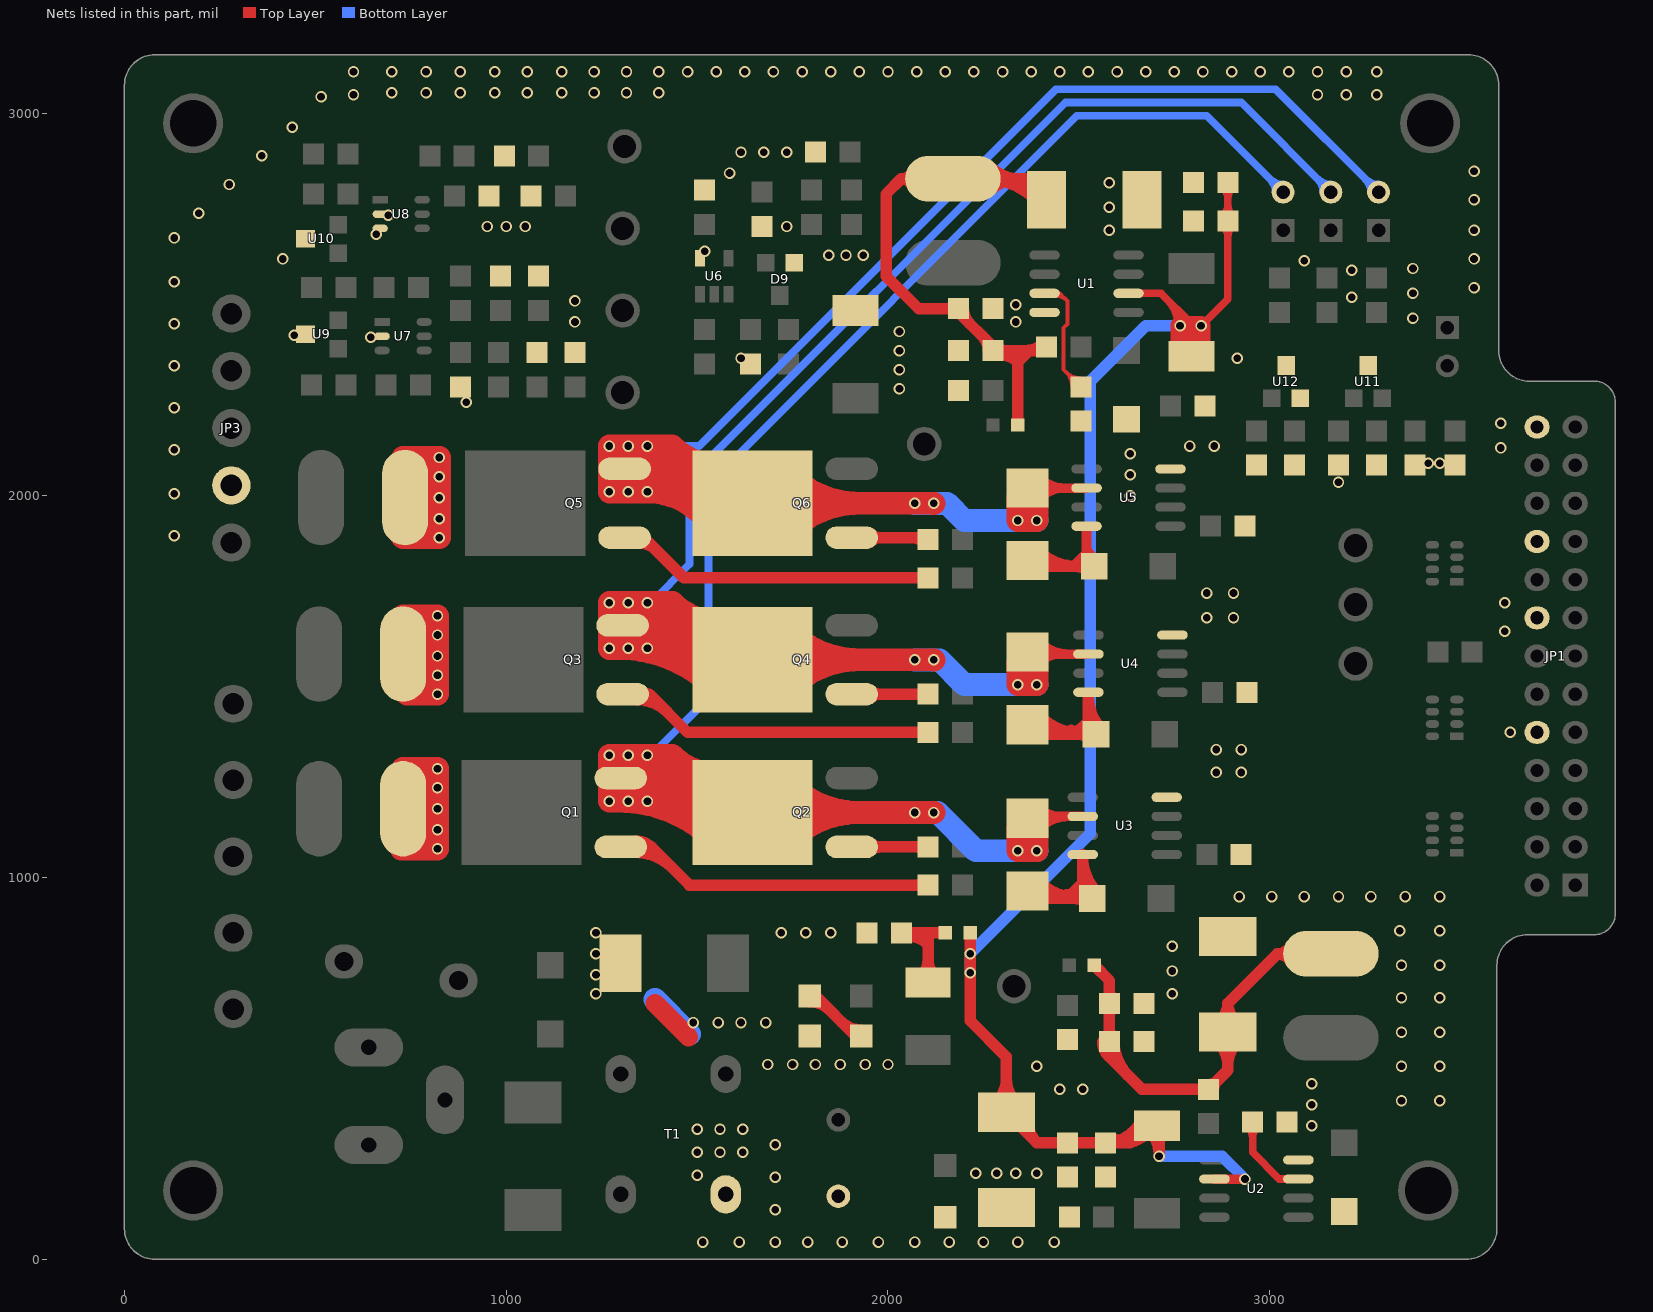
[diagram p0: the nets of this part, all layers, seen from the top]
# Altium PCB MISC103926.PcbDoc (part 2 of 4)
Units mil, origin at the board's own origin, x right, y up, seen from the top; angles counter-clockwise.
Board outline 3905 x 3155 mil, 4 copper layers (Top Layer, GND1, GND2, Bottom Layer); 132 components, 84 nets, 362 pads, 268 vias.

## Via types
v1: diameter 30, hole 20, Top Layer to Bottom Layer, 268 vias

## Nets (pads, with @x,y where several pads share a name; then routed paths per layer and width w, separated by ;. In a path a pad name is that pad's centre, name@x,y a point inside that pad or via, vN(x,y) a via of type N, cw(c..) or ccw(c..) an arc to the next point about the centre after c; other vN are vias at no path point) (continued)
GND: C2.2 C3.2 C4.2 C5.2 C6.2 C7.2 C8.2 C9.2 C10.2 C11.2 C12.2 C13.2 C14.2 C15.2 C16.2 C17.2 C19.2 C20.1 C21.1 C22.1 C26.1 C27.1 C28.2 C29.2 C30.2 C31.1 C32.2 C33.2 C34.2 C35.1 C36.1 C37.1 D3.2 D4.2 D5.2 D9.1 D10.2 JP1.10 JP1.16 JP1.20 JP1.26 JP3.2 R3.2 R5.2 R16.2 R19.1 R20.1 R21.1 R22.1 R32.2 R33.2 R34.2 T1.2 U1.4 U2.4 U3.4 U4.4 U5.4 U6.5 U7.2 U8.2 U8.3 U9.3 U10.3 U11.3 U12.2 U12.3 | length 352.7
  Top Layer w10: v1(645,2415) 647.6,2417.6 U7.2@675,2417.6 ccw(c675,2385.58) v1@652.14,2408 ; v1@652.07,2422.07 ccw(c662.87,2432.87) U7.2@662.87,2417.6 ; U7.2@661.46,2414.06 ccw(c652.93,2405.53) 652.93,2417.6 ccw(c652.93,2429.67) U7.2@661.46,2421.13
  Top Layer w50: 1390,670 1477.5,582.5
  Top Layer w60: C5.2@2285,125 C5.2@2295,135
  Bottom Layer w60: 1390,680 1480,590
  other v1: 1515,45 1610,45 1705,45 1790,45 1880,45 1975,45 2070,45 2160,45 2250,45 2340,45 2435,45 1705,130 1705,215 1500,220 2230,225 2285,225 2335,225 2390,225 1500,280 1560,280 1620,280 1705,300 1500,340 1560,340 1620,340 3110,350 3110,405 3345,415 3445,415 2450,445 2510,445 3110,460 2390,505 3345,505 3445,505 1685,510 1750,510 1810,510 1875,510 1940,510 2000,510 3345,595 3445,595 1490,620 1555,620 1615,620 1680,620 3345,685 3445,685 1235,695 2745,695 1235,745 2745,755 3345,770 3445,770 1235,800 2745,820 1235,855 1720,855 1785,855 1850,855 3340,860 3445,860 2920,950 3005,950 3090,950 3180,950 3265,950 3355,950 3445,950 2860,1275 2925,1275 2860,1335 2925,1335 3630,1380 3615,1645 2835,1680 2905,1680 3615,1720 2835,1745 2905,1745 130,1895 2635,2000 130,2005 3180,2035 2635,2055 3415,2085 3445.5,2085 2635,2110 130,2120 3605,2125 2790,2130 2855,2130 3605,2190 130,2230 895,2245 2030,2280 2030,2330 130,2340 1615,2360 2915,2360 2030,2380 445,2420 2030,2430 130,2450 1180,2455 2335,2455 3375,2465 2335,2500 1180,2510 3215,2520 3375,2530 3535,2545 130,2560 3215,2590 3375,2595 3090,2615 415,2620 3535,2620 1845,2630 1890,2630 1935,2630 1520,2640 130,2675 660,2685 2580,2695 3535,2695 950,2705 1000,2705 1050,2705 1735,2705 690.87,2734.06 195,2740 2580,2755 3535,2775 275,2815 2580,2820 1585,2845 3535,2850 360,2890 1615,2900 1675,2900 1735,2900 440,2965 515,3045 600,3050 3125,3050 3200,3050 3280,3050 700,3055 790,3055 880,3055 970,3055 1055,3055 1145,3055 1230,3055 1315,3055 1400,3055 600,3110 700,3110 790,3110 880,3110 970,3110 1055,3110 1145,3110 1230,3110 1315,3110 1400,3110 1475,3110 1550,3110 1625,3110 1700,3110 1775,3110 1850,3110 1925,3110 2000,3110 2075,3110 2150,3110 2225,3110 2300,3110 2375,3110 2450,3110 2525,3110 2600,3110 2675,3110 2750,3110 2825,3110 2900,3110 2975,3110 3050,3110 3125,3110 3200,3110 3280,3110
GT_UH: Q1.1 R9.2 | length 1101.2
  Top Layer w30: Q1.1@1300,1080 1380,1080 1480,980 R9.2@2105,980 ; Q1.1@1339.37,1065.47 cw(c1339.37,932.31) 1433.53,1026.47 ; Q1.1@1339.37,1095.47 cw(c1339.37,1034.73) 1382.32,1077.68 ; Q1.1@1349.64,1069.73 cw(c1374.44,1044.93) 1374.44,1080 cw(c1374.44,1115.07) Q1.1@1349.64,1090.27 ; R9.2@2096.16,971.16 ccw(c2074.82,949.82) 2074.82,980 ccw(c2074.82,1010.18) R9.2@2096.16,988.84
GT_UL: Q2.1 R10.2 | length 302.5
  Top Layer w30: Q2.1@1905,1080 R10.2@2105,1080 ; Q2.1@1954.64,1069.73 cw(c1979.44,1044.93) 1979.44,1080 cw(c1979.44,1115.07) Q2.1@1954.64,1090.27 ; R10.2@2096.16,1071.16 ccw(c2074.82,1049.82) 2074.82,1080 ccw(c2074.82,1110.18) R10.2@2096.16,1088.84
GT_VH: Q3.1 R11.2 | length 1018.8
  Top Layer w30: Q3.1@1305,1480 1375,1480 ; Q3.1@1344.37,1465.47 cw(c1344.37,1356.45) 1421.46,1433.54 ; Q3.1@1355.62,1470.81 cw(c1375,1454.97) 1375,1480 ; Q3.1@1355.62,1489.19 ccw(c1375,1505.02) 1375,1480 ; R11.2@2096.16,1371.16 ccw(c2074.82,1349.82) 2074.82,1380 ccw(c2074.82,1410.18) R11.2@2096.16,1388.84 ; R11.2@2105,1380 1475,1380 1375,1480
GT_VL: Q4.1 R12.2 | length 302.5
  Top Layer w30: Q4.1@1905,1480 R12.2@2105,1480 ; Q4.1@1954.64,1469.73 cw(c1979.44,1444.93) 1979.44,1480 cw(c1979.44,1515.07) Q4.1@1954.64,1490.27 ; R12.2@2096.16,1471.16 ccw(c2074.82,1449.82) 2074.82,1480 ccw(c2074.82,1510.18) R12.2@2096.16,1488.84
GT_WH: Q5.1 R13.2 | length 933.6
  Top Layer w30: Q5.1@1310,1890 1360,1890 1465,1785 R13.2@2105,1785 ; Q5.1@1349.37,1875.47 cw(c1349.37,1814.73) 1392.32,1857.68 ; R13.2@2096.16,1776.16 ccw(c2074.82,1754.82) 2074.82,1785 ccw(c2074.82,1815.18) R13.2@2096.16,1793.84
GT_WL: Q6.1 R14.2 | length 294.3
  Top Layer w20: R14.2@2100,1890 R14.2@2105,1885
  Top Layer w30: Q6.1@1905,1890 R14.2@2100,1890 ; Q6.1@1954.64,1879.73 cw(c1979.44,1854.93) 1979.44,1890 cw(c1979.44,1925.07) Q6.1@1954.64,1900.27 ; 2062.75,1890 cw(c2062.75,1842.75) R14.2@2096.16,1876.16
MT_PU: C23.2 J1.2 L6.1 Q1.3 Q2.2 U3.6 | length 9709.6
  Top Layer w25: C23.2@2370,1160 U3.6@2510,1160 ; C23.2@2396.29,1127.65 cw(c2474.39,1049.54) U3.6@2474.39,1160 ; C23.2@2396.29,1182.35 ccw(c2450.25,1236.31) 2450.25,1160
  Top Layer w50: C23.2@2340,1130 C23.2@2365,1155 C23.2@2390,1130
  Top Layer w60: L6.1@725,1075 v1(820,1075) ; L6.1@730,1285 v1(820,1285) ; L6.1@743.07,1088 cw(c772.39,1027.4) v1(820,1075) ; L6.1@743.07,1272 ccw(c772.4,1332.6) v1(820,1285) ; L6.1@751.21,1158.79 cw(c802.43,1107.57) 802.43,1180 cw(c802.43,1252.43) L6.1@751.21,1201.21 ; L6.1@759.08,1122.38 ccw(c820,1137.85) v1(820,1075) ; L6.1@759.08,1237.62 cw(c820,1222.15) v1(820,1285) ; L6.1@760.25,1134.75 ccw(c820,1194.5) 820,1110 ; L6.1@760.25,1225.25 cw(c820,1165.5) 820,1250 ; 805.5,1128.85 ccw(c859.51,1114.51) v1(820,1075) ; 805.5,1231.15 cw(c859.51,1245.49) v1(820,1285) ; 805.74,1175.33 cw(c861.43,1193.56) v1(820,1235) L6.1@765,1180 ; 805.74,1184.67 ccw(c861.43,1166.44) v1(820,1125) L6.1@765,1180 ; v1(820,1180) L6.1@730,1180 ; 1293.03,1200 cw(c1293.03,837.87) Q2.2@1549.09,1093.93 ; Q1.3@1309.68,1260.32 Q1.3@1300,1260.32 Q1.3@1310.32,1260.32 ; v1(1320,1200) v1(1320,1320) ; v1@1320,1214.69 cw(c1384.99,1214.69) Q1.3@1339.04,1260.65 ; v1@1320,1305.94 ccw(c1384.99,1305.94) Q1.3@1339.04,1259.98 ; Q1.3@1339.65,1259.93 ccw(c1295.39,1320) v1(1370,1320) ; Q1.3@1339.69,1260.67 cw(c1278.59,1192.67) v1@1370,1192.67 ; 1437.12,1200 ccw(c1437.12,1358.35) Q2.2@1549.09,1246.38 ; 1437.88,1200 cw(c1437.88,982.72) Q2.2@1591.52,1136.36 ; 1469.92,1285.08 cw(c1354.99,1170.16) Q2.2@1517.52,1170.16 ; Q2.2@1540,1215 1435,1320 ; Q2.2@1575.16,1170.16 Q2.2@1645,1170.16 ; Q2.2@1599.02,1274.7 cw(c1556.94,1441.93) 1435.01,1319.99 ; Q2.2@1740.91,1093.93 cw(c1924.93,909.92) 1924.93,1170.16 cw(c1924.93,1430.4) Q2.2@1740.91,1246.38 ; v1(2120,1170) 2119.84,1170.16 Q2.2@1645,1170.16 ; C23.2@2340,1130 v1(2340,1070) v1(2390,1070) C23.2@2390,1130 ; L6.1@730,1180 730,1195 v1(820,1285) ; L6.1@730,1180 L6.1@765,1180 ; L6.1@730,1180 730,1165 v1(820,1075) ; L6.1@730,1180 L6.1@765,1180 ; v1(820,1075) v1(820,1285) ; v1(1270,1200) v1(1370,1200) v1(1370,1320) ; v1(1270,1200) v1(1270,1320) v1(1370,1320) ; v1(1270,1200) 1615.16,1200 Q2.2@1645,1170.16 ; v1(1370,1320) 1435,1320
  Top Layer w70: 1418.03,1260.32 cw(c1418.03,1056.9) Q2.2@1596.54,1154.43 ; Q2.2@1535.11,1120.87 ccw(c1300.01,992.42) Q1.3@1300,1260.32 1554.84,1260.32 Q2.2@1645,1170.16
  Bottom Layer w20: v1(1370,1320) 1380,1320 1530,1470 1530,2030 2495,2995 2835,2995 J1.2@3035,2795 ; J1.2@3015,2795 ccw(c2966.72,2795) 3000.86,2829.14 ccw(c3035,2863.28) J1.2@3035,2815
  Bottom Layer w60: v1(2070,1170) 2130,1170 2230,1070 v1(2390,1070)
MT_PV: C24.2 J2.2 L7.1 Q3.3 Q4.2 U4.6 | length 9255.4
  Top Layer w25: C24.2@2370,1585 U4.6@2525,1585 ; C24.2@2396.29,1562.65 cw(c2450.25,1508.69) 2450.25,1585 ; C24.2@2396.29,1617.35 ccw(c2474.39,1695.45) 2474.39,1585
  Top Layer w60: L7.1@715,1670 730,1685 v1(820,1685) ccw(c820,1620.2) L7.1@758.48,1640.57 ; L7.1@740,1480 v1(820,1480) ; L7.1@743.07,1493 cw(c772.39,1432.4) v1(820,1480) ; L7.1@747.62,1674.28 ccw(c780.46,1719.54) v1@820,1680 ; L7.1@751.21,1563.79 cw(c802.43,1512.57) 802.43,1585 cw(c802.43,1657.43) L7.1@751.21,1606.21 ; L7.1@759.08,1527.38 ccw(c820,1542.85) v1(820,1480) ; L7.1@760.25,1539.75 ccw(c820,1599.5) 820,1515 ; L7.1@768.79,1628.79 cw(c820,1577.57) 820,1650 ; 805.26,1632.21 cw(c857.83,1642.16) v1@820,1680 ; 805.5,1533.85 ccw(c859.51,1519.51) v1(820,1480) ; 805.5,1576.15 cw(c859.51,1590.49) 820,1630 775,1585 L7.1@730,1585 ; 805.5,1583.85 ccw(c859.51,1569.51) v1(820,1530) 765,1585 L7.1@730,1585 ; v1(820,1580) 815,1585 L7.1@730,1585 ; 1293.03,1600 cw(c1293.03,1237.87) Q4.2@1549.09,1493.93 ; Q3.3@1305,1660.32 Q3.3@1310.32,1660.32 ; Q3.3@1305.33,1659.98 ccw(c1269.93,1695.39) 1320,1695.39 ; Q3.3@1305.33,1660.65 cw(c1269.93,1625.24) 1320,1625.24 ; v1(1320,1600) v1(1320,1720) ; Q3.3@1344.7,1659.98 ccw(c1286.16,1720) v1(1370,1720) ; Q3.3@1344.7,1660.65 cw(c1283.64,1599.58) v1@1370,1599.58 ; 1437.12,1600 ccw(c1437.12,1758.35) Q4.2@1549.09,1646.38 ; 1437.88,1600 cw(c1437.88,1382.72) Q4.2@1591.52,1536.36 ; 1469.69,1685.62 cw(c1354.23,1570.16) Q4.2@1517.52,1570.16 ; Q4.2@1495,1660.32 1435.32,1720 ; Q4.2@1599.08,1674.71 cw(c1557.15,1841.82) 1435.32,1719.99 ; Q4.2@1740.91,1493.93 cw(c1924.93,1309.92) 1924.93,1570.16 cw(c1924.93,1830.4) Q4.2@1740.91,1646.38 ; v1(2120,1570) 2119.84,1570.16 Q4.2@1645,1570.16 1615.16,1600 v1(1270,1600) ; L7.1@730,1585 730,1590 v1@820,1680 ; L7.1@730,1585 730,1570 v1(820,1480) ; v1(820,1480) v1@820,1680 ; v1(1270,1600) v1(1370,1600) v1(1370,1720) ; v1(1270,1600) v1(1270,1720) v1(1370,1720) ; v1(1370,1720) 1435.32,1720 ; v1(2340,1505) 2340,1565 C24.2@2365,1590 2390,1565 v1(2390,1505) v1(2340,1505)
  Top Layer w70: 1421.21,1660.32 cw(c1421.21,1462.23) Q4.2@1596.32,1554.83 ; Q4.2@1534.44,1522.1 ccw(c1305.01,1400.78) Q3.3@1305,1660.32 1554.84,1660.32 Q4.2@1645,1570.16
  Bottom Layer w20: v1(1370,1720) 1380,1720 1480,1820 1480,2045 2465,3030 2925,3030 J2.2@3160,2795 ; J2.2@3140,2795 ccw(c3091.72,2795) 3125.86,2829.14 ccw(c3160,2863.28) J2.2@3160,2815
  Bottom Layer w60: v1(2070,1570) 2135,1570 2200,1505 v1(2390,1505)
  other v1: 820,1635
MT_PW: C25.2 J3.2 L8.1 Q5.3 Q6.2 U5.6 | length 8872.7
  Top Layer w25: C25.2@2365,2020 U5.6@2520,2020 ; C25.2@2396.29,1992.65 cw(c2462.32,1926.62) 2462.32,2020 cw(c2462.32,2113.38) C25.2@2396.29,2047.35
  Top Layer w60: L8.1@725,1895 730,1890 v1(825,1890) ; L8.1@730,2100 v1(825,2100) ; L8.1@748.07,1903 cw(c777.39,1842.4) v1(825,1890) ; L8.1@748.07,2087 ccw(c777.4,2147.6) v1(825,2100) ; L8.1@756.21,1973.79 cw(c807.43,1922.57) 807.43,1995 cw(c807.43,2067.43) L8.1@756.21,2016.21 ; L8.1@764.08,1937.38 ccw(c825,1952.85) v1(825,1890) ; L8.1@764.08,2052.62 cw(c825,2037.15) v1(825,2100) ; L8.1@765.25,1949.75 ccw(c825,2009.5) 825,1925 ; L8.1@765.25,2040.25 cw(c825,1980.5) 825,2065 ; 810.5,1943.85 ccw(c864.51,1929.51) v1(825,1890) ; 810.5,2046.15 cw(c864.51,2060.49) v1(825,2100) ; 810.74,1990.33 cw(c866.43,2008.56) v1(825,2050) L8.1@770,1995 ; 810.74,1999.67 ccw(c866.43,1981.44) v1(825,1940) L8.1@770,1995 ; v1(825,1995) L8.1@735,1995 ; Q5.3@1319.68,2070.32 Q5.3@1310,2070.32 Q5.3@1320.32,2070.32 ; v1(1320,2010) v1(1320,2130) ; Q5.3@1349.7,2069.98 ccw(c1300.71,2118.98) v1@1370,2118.98 ; Q5.3@1349.7,2070.65 cw(c1300.71,2021.65) v1@1370,2021.65 ; 1437.12,2010 ccw(c1437.12,2168.35) Q6.2@1549.09,2056.38 ; 1469.92,2095.08 cw(c1354.99,1980.16) Q6.2@1517.52,1980.16 ; 1481.3,2010 cw(c1481.3,1885.41) Q6.2@1585.39,1953.89 ; Q6.2@1535.26,1920.91 ccw(c1370.01,1812.19) v1(1370,2010) ; Q6.2@1554.84,2070.32 Q6.2@1645,1980.16 ; Q6.2@1555,2010 1435,2130 ; Q6.2@1599.02,2084.7 cw(c1556.94,2251.93) 1435.01,2129.99 ; Q6.2@1740.91,1903.93 cw(c1924.93,1719.92) 1924.93,1980.16 cw(c1924.93,2240.4) Q6.2@1740.91,2056.38 ; v1(2120,1980) 2119.84,1980.16 Q6.2@1645,1980.16 ; L8.1@735,1995 735,2010 v1(825,2100) ; L8.1@735,1995 L8.1@770,1995 ; L8.1@735,1995 735,1980 v1(825,1890) ; L8.1@735,1995 L8.1@770,1995 ; v1(825,1890) v1(825,2100) ; v1(1320,2130) v1(1270,2130) v1(1270,2010) v1(1370,2010) ; v1(1320,2130) v1(1370,2130) ; v1(1370,2010) 1615.16,2010 Q6.2@1645,1980.16 ; v1(1370,2010) 1370,2070.32 v1(1370,2130) ; v1(1370,2130) 1435,2130 ; v1(2340,1935) 2340,1995 C25.2@2365,2020 2390,1995 v1(2390,1935) v1(2340,1935)
  Top Layer w70: Q5.3@1310,2070.32 cw(c1310.01,1819.02) Q6.2@1533.78,1933.38 ; Q5.3@1319.68,2070.32 1320.32,2070.32 1370,2070.32 Q6.2@1490,2070.32 ; 1424.4,2070.32 cw(c1424.4,1877.48) Q6.2@1596.11,1965.23
  Bottom Layer w20: v1(1370,2130) 1430,2130 ; 1400,2105 1405,2105 1430,2130 ; J3.2@3265,2795 ccw(c3216.72,2795) 3250.86,2829.14 ccw(c3285,2863.28) J3.2@3285,2815 ; J3.2@3285,2795 3015,3065 2440,3065 1505,2130 1430,2130
  Bottom Layer w60: v1(2070,1980) 2155,1980 2200,1935 v1(2390,1935)
NetC1_2: C1.2 C2.1 | length 292.3
  Top Layer w30: C1.2@1795,675 cw(c1795,602.57) 1846.21,653.79 ; C1.2@1795,690 1810,690 1915,585 C2.1@1930,585 ; 1878.79,621.21 ccw(c1930,672.42) C2.1@1930,600
NetC3_1: C3.1 F1.2 L1.1 | length 579.4
  Top Layer w30: C3.1@2035,855 L1.1@2140,855 ; C3.1@2038.23,842.92 cw(c2056.08,776.08) 2105,825 ; 2075,855 2105,825 ; F1.2@2087.77,742.23 ccw(c2046.17,783.83) 2105,783.83 ccw(c2163.84,783.83) F1.2@2122.23,742.23 ; F1.2@2105,725 2105,825 ; 2105,850 2105,825 ; C3.1@2043.84,846.16 cw(c2065.18,824.82) 2065.18,855 ; C3.1@2043.84,846.16 cw(c2065.18,824.82) 2065.18,855 ; C3.1@2043.84,846.16 cw(c2065.18,824.82) 2065.18,855 ; C3.1@2043.84,863.84 ccw(c2065.18,885.18) 2065.18,855 ; C3.1@2043.84,863.84 ccw(c2065.18,885.18) 2065.18,855 ; C3.1@2043.84,863.84 ccw(c2065.18,885.18) 2065.18,855
NetC4_1: C4.1 C5.1 C6.1 C7.1 C8.1 L1.2 R2.1 R4.1 U1.6 U2.6 | length 5738.5
  Top Layer w20: C5.1@2310,385 C5.1@2330,405 ; U1.6@2630,2530 2715,2530 2795,2450 R2.1@2795,2365 R2.1@2815,2365 ; R4.1@2692.5,362.5 R4.1@2710,345 ; 2731.72,2513.28 cw(c2663.43,2445) v1@2760,2445 ; 2765.86,2479.14 cw(c2731.72,2445) 2780,2445 ; R2.1@2773.79,2386.21 ccw(c2722.57,2437.43) 2795,2437.43 ccw(c2867.43,2437.43) R2.1@2816.21,2386.21 ; v1(2820,2445) 2890,2515 C6.1@2890,2720 C4.1@2890,2820 ; C6.1@2877.63,2707.63 cw(c2847.75,2677.75) 2890,2677.75 cw(c2932.25,2677.75) C6.1@2902.37,2707.63 ; C6.1@2877.63,2732.37 ccw(c2847.75,2762.25) 2890,2762.25 ccw(c2932.25,2762.25) C6.1@2902.37,2732.37 ; C4.1@2877.63,2807.63 cw(c2847.75,2777.75) 2890,2777.75 cw(c2932.25,2777.75) C4.1@2902.37,2807.63
  Top Layer w25: U2.6@2855,210 v1(2935,210)
  Top Layer w30: L1.2@2215,855 2215,625 2310,530 C5.1@2310,385 2390,305 ; C5.1@2284.42,410.58 ccw(c2222.65,472.35) 2310,472.35 ccw(c2397.35,472.35) C5.1@2335.58,410.58 ; C5.1@2368.95,377.18 ccw(c2445.28,360.28) 2390,305 ; C7.1@2461.16,296.16 ccw(c2439.82,274.82) 2439.82,305 ccw(c2439.82,335.18) C7.1@2461.16,313.84 ; C7.1@2478.84,296.16 cw(c2500.18,274.82) 2500.18,305 cw(c2500.18,335.18) C7.1@2478.84,313.84 ; C8.1@2561.16,296.16 ccw(c2539.82,274.82) 2539.82,305 ccw(c2539.82,335.18) C8.1@2561.16,313.84 ; C8.1@2576.25,315.83 ccw(c2591.34,341.96) 2599.15,312.81 ccw(c2606.96,283.66) C8.1@2580.83,298.75 ; C8.1@2578.84,296.16 cw(c2600.18,274.82) 2600.18,305 cw(c2600.18,335.18) C8.1@2578.84,313.84 ; 2619.29,305 ccw(c2619.29,383.98) R4.1@2689.44,347.7 ; R4.1@2645.86,315.86 ccw(c2611.72,350) R4.1@2660,350 ; R4.1@2662.79,361.48 cw(c2570,409.46) C8.1@2570,305 ; R4.1@2684.55,325 ccw(c2683.32,256.69) 2635,305 ; R4.1@2687.32,332.32 cw(c2632.58,277.58) v1@2710,277.58 ; R4.1@2692.5,362.5 2635,305 ; v1(2710,270) R4.1@2710,345 ; 2710,301.71 cw(c2753.29,301.71) R4.1@2722.68,332.32 ; 2390,305 C7.1@2470,305 C8.1@2570,305 ; C8.1@2570,305 2635,305
  Top Layer w50: 2765,2425.35 ccw(c2835.35,2425.35) R2.1@2785.61,2375.61 ; R2.1@2795,2365 2765,2395 v1(2765,2445) v1(2820,2445) 2820,2370 R2.1@2815,2365 ; R2.1@2804.39,2375.61 ccw(c2766.71,2413.29) 2820,2413.29
  Bottom Layer w30: v1(2215,750) v1(2215,800) 2530,1115 2530,2300 2675,2445 v1(2820,2445) ; v1(2710,270) 2875,270 v1(2935,210)
NetC9_1: C9.1 U1.3 | length 501.1
  Top Layer w10: U1.3@2410,2530 2450,2530 2470,2510 ; U1.3@2437.96,2533 cw(c2438.22,2511.8) 2453.21,2526.79 ; U1.3@2438.08,2523 cw(c2438.61,2478.61) 2470,2510 ; C9.1@2482.5,2285 ccw(c2428.18,2285) 2466.59,2323.41 ccw(c2505,2361.82) C9.1@2505,2307.5 ; C9.1@2492.5,2285 ccw(c2462.32,2285) 2483.66,2306.34 ccw(c2505,2327.68) C9.1@2505,2297.5 ; C9.1@2505,2285 2460,2330 2460,2440 2470,2450 2470,2510
NetC10_1: C10.1 U2.3 | length 295.4
  Top Layer w20: C10.1@2942.63,347.63 cw(c2912.75,317.75) 2955,317.75 cw(c2997.25,317.75) C10.1@2967.37,347.63 ; C10.1@2955,360 2955,280 3025,210 U2.3@3075,210
NetC11_1: C11.1 C12.1 C14.1 L2.2 L4.1 R6.2 | length 2338.3
  Top Layer w30: L2.2@2064.06,2811.32 ccw(c2035,2798.06) 2035,2830 ; L2.2@2064.06,2848.68 cw(c2035,2861.94) 2035,2830 ; C14.1@2176.16,2481.16 ccw(c2154.82,2459.82) 2154.82,2490 ccw(c2154.82,2520.18) C14.1@2176.16,2498.84 ; C14.1@2197.5,2490 ccw(c2251.82,2490) 2213.41,2451.59 ; 2246.59,2418.41 cw(c2208.18,2380) C12.1@2262.5,2380 ; L2.2@2251.9,2830 cw(c2251.9,2635.52) C11.1@2389.42,2773.04 ; L2.2@2266.82,2798.18 cw(c2343.64,2721.36) 2343.64,2830 cw(c2343.64,2938.64) L2.2@2266.82,2861.82 ; C12.1@2277.82,2367.82 cw(c2292.84,2302.84) 2340,2350 ; 2310,2380 2340,2350 ; 2324.32,2830 cw(c2324.32,2707.95) C11.1@2410.63,2794.25 ; L4.1@2340,2185 2340,2350 ; 2340,2380 2340,2350 ; 2360.68,2380 ccw(c2360.68,2444.32) R6.2@2406.16,2398.84 ; 2370,2380 2340,2350 ; R6.2@2415,2390 2405,2380 C12.1@2275,2380 2275,2390 2185,2480 C14.1@2185,2490 2080,2490 1995,2575 1995,2790 2035,2830 ; C11.1@2420,2830 L2.2@2170,2830 2035,2830 ; C12.1@2283.84,2371.16 cw(c2305.18,2349.82) 2305.18,2380 ; C12.1@2283.84,2371.16 cw(c2305.18,2349.82) 2305.18,2380 ; C12.1@2283.84,2371.16 cw(c2305.18,2349.82) 2305.18,2380 ; C12.1@2283.84,2388.84 ccw(c2305.18,2410.18) 2305.18,2380 ; C12.1@2283.84,2388.84 ccw(c2305.18,2410.18) 2305.18,2380 ; C12.1@2283.84,2388.84 ccw(c2305.18,2410.18) 2305.18,2380
NetC13_1: C13.1 C15.1 C16.1 L3.2 L5.1 R7.2 | length 1878.9
  Top Layer w30: L5.1@2540,770 2580,730 C15.1@2580,570 2580,530 2665,445 R7.2@2840,445 2890,495 C13.1@2890,595 2890,670 ; C15.1@2562.5,570 ccw(c2616.82,570) 2578.41,531.59 ; C15.1@2571.16,561.16 cw(c2549.82,539.82) 2580,539.82 cw(c2610.18,539.82) C15.1@2588.84,561.16 ; C15.1@2571.16,578.84 ccw(c2549.82,600.18) 2580,600.18 ccw(c2610.18,600.18) C15.1@2588.84,578.84 ; C16.1@2571.16,661.16 cw(c2549.82,639.82) 2580,639.82 cw(c2610.18,639.82) C16.1@2588.84,661.16 ; C16.1@2571.16,678.84 ccw(c2549.82,700.18) 2580,700.18 ccw(c2610.18,700.18) C16.1@2588.84,678.84 ; C15.1@2592.5,570 ccw(c2719.25,570) 2629.62,480.38 ; R7.2@2831.16,436.16 ccw(c2809.82,414.82) 2809.82,445 ccw(c2809.82,475.18) R7.2@2831.16,453.84 ; R7.2@2840,457.5 ccw(c2840,487.68) 2861.34,466.34 ccw(c2882.68,445) R7.2@2852.5,445 ; C13.1@2864.42,569.42 cw(c2802.65,507.65) 2890,507.65 cw(c2977.35,507.65) C13.1@2915.58,569.42 ; C13.1@2867.48,623.32 ccw(c2830.36,670) 2890,670 ; C13.1@2912.52,623.32 cw(c2949.64,670) 2890,670 ; L3.2@3055.29,778.82 ccw(c3020,760) 3020,800 ; L3.2@3055.29,821.18 cw(c3020,840) 3020,800 ; L3.2@3160,800 3020,800 ; 2890,670 3020,800
NetC23_1: C23.1 D6.1 U3.8 | length 833.6
  Top Layer w30: C23.1@2365,965 2385,945 D6.1@2535,945 2510,970 2510,985 ; C23.1@2373.31,969.37 ccw(c2432.14,1028.21) 2432.14,945 ; C23.1@2394.52,990.58 ccw(c2504.57,1100.63) D6.1@2504.57,945 ; 2467.96,954.81 ccw(c2487.41,1027.42) D6.1@2525,962.32 ; 2475,945 2475,950 2510,985 ; 2510,981.21 ccw(c2571.21,981.21) D6.1@2527.93,937.93 ; U3.8@2510,1053.64 ccw(c2643.64,1053.64) D6.1@2549.14,959.14 ; U3.8@2510,1060 2510,985 ; D6.1@2520.86,930.86 ccw(c2486.72,896.72) 2486.72,945 ccw(c2486.72,993.28) D6.1@2520.86,959.14
NetC24_1: C24.1 D7.1 U4.8 | length 789.1
  Top Layer w30: C24.1@2365,1400 2390,1375 D7.1@2545,1375 2525,1395 2525,1415 ; C24.1@2373.31,1404.37 ccw(c2444.21,1475.28) 2444.21,1375 ; C24.1@2394.52,1425.58 ccw(c2516.64,1547.7) D7.1@2516.64,1375 ; 2479.35,1384.99 ccw(c2498.33,1455.84) D7.1@2535,1392.32 ; 2490,1375 2525,1410 2525,1415 ; D7.1@2530.86,1360.86 ccw(c2496.72,1326.72) 2496.72,1375 ccw(c2496.72,1423.28) D7.1@2530.86,1389.14 ; D7.1@2559.14,1389.14 cw(c2641.56,1471.56) 2525,1471.56 2525,1415
NetC25_1: C25.1 D8.1 U5.8 | length 664.2
  Top Layer w25: 2470,1815 2470,1820 ; 2485,1815 2520,1850 2520,1855 ; U5.8@2520,1920 2520,1870 ; D8.1@2540,1815 2520,1835 2520,1855 ; D8.1@2545.68,1836.77 cw(c2554.34,1870) 2520,1870 ; 2520,1855 2520,1870
  Top Layer w30: C25.1@2365,1830 2380,1815 D8.1@2540,1815 ; C25.1@2373.31,1834.37 ccw(c2420.07,1881.14) 2420.07,1815 ccw(c2420.07,1778.86) C25.1@2394.52,1804.42 ; C25.1@2394.52,1855.58 ccw(c2492.5,1953.56) 2492.5,1815 ; D8.1@2525.86,1800.86 ccw(c2491.72,1766.72) 2491.72,1815 ccw(c2491.72,1863.28) D8.1@2525.86,1829.14